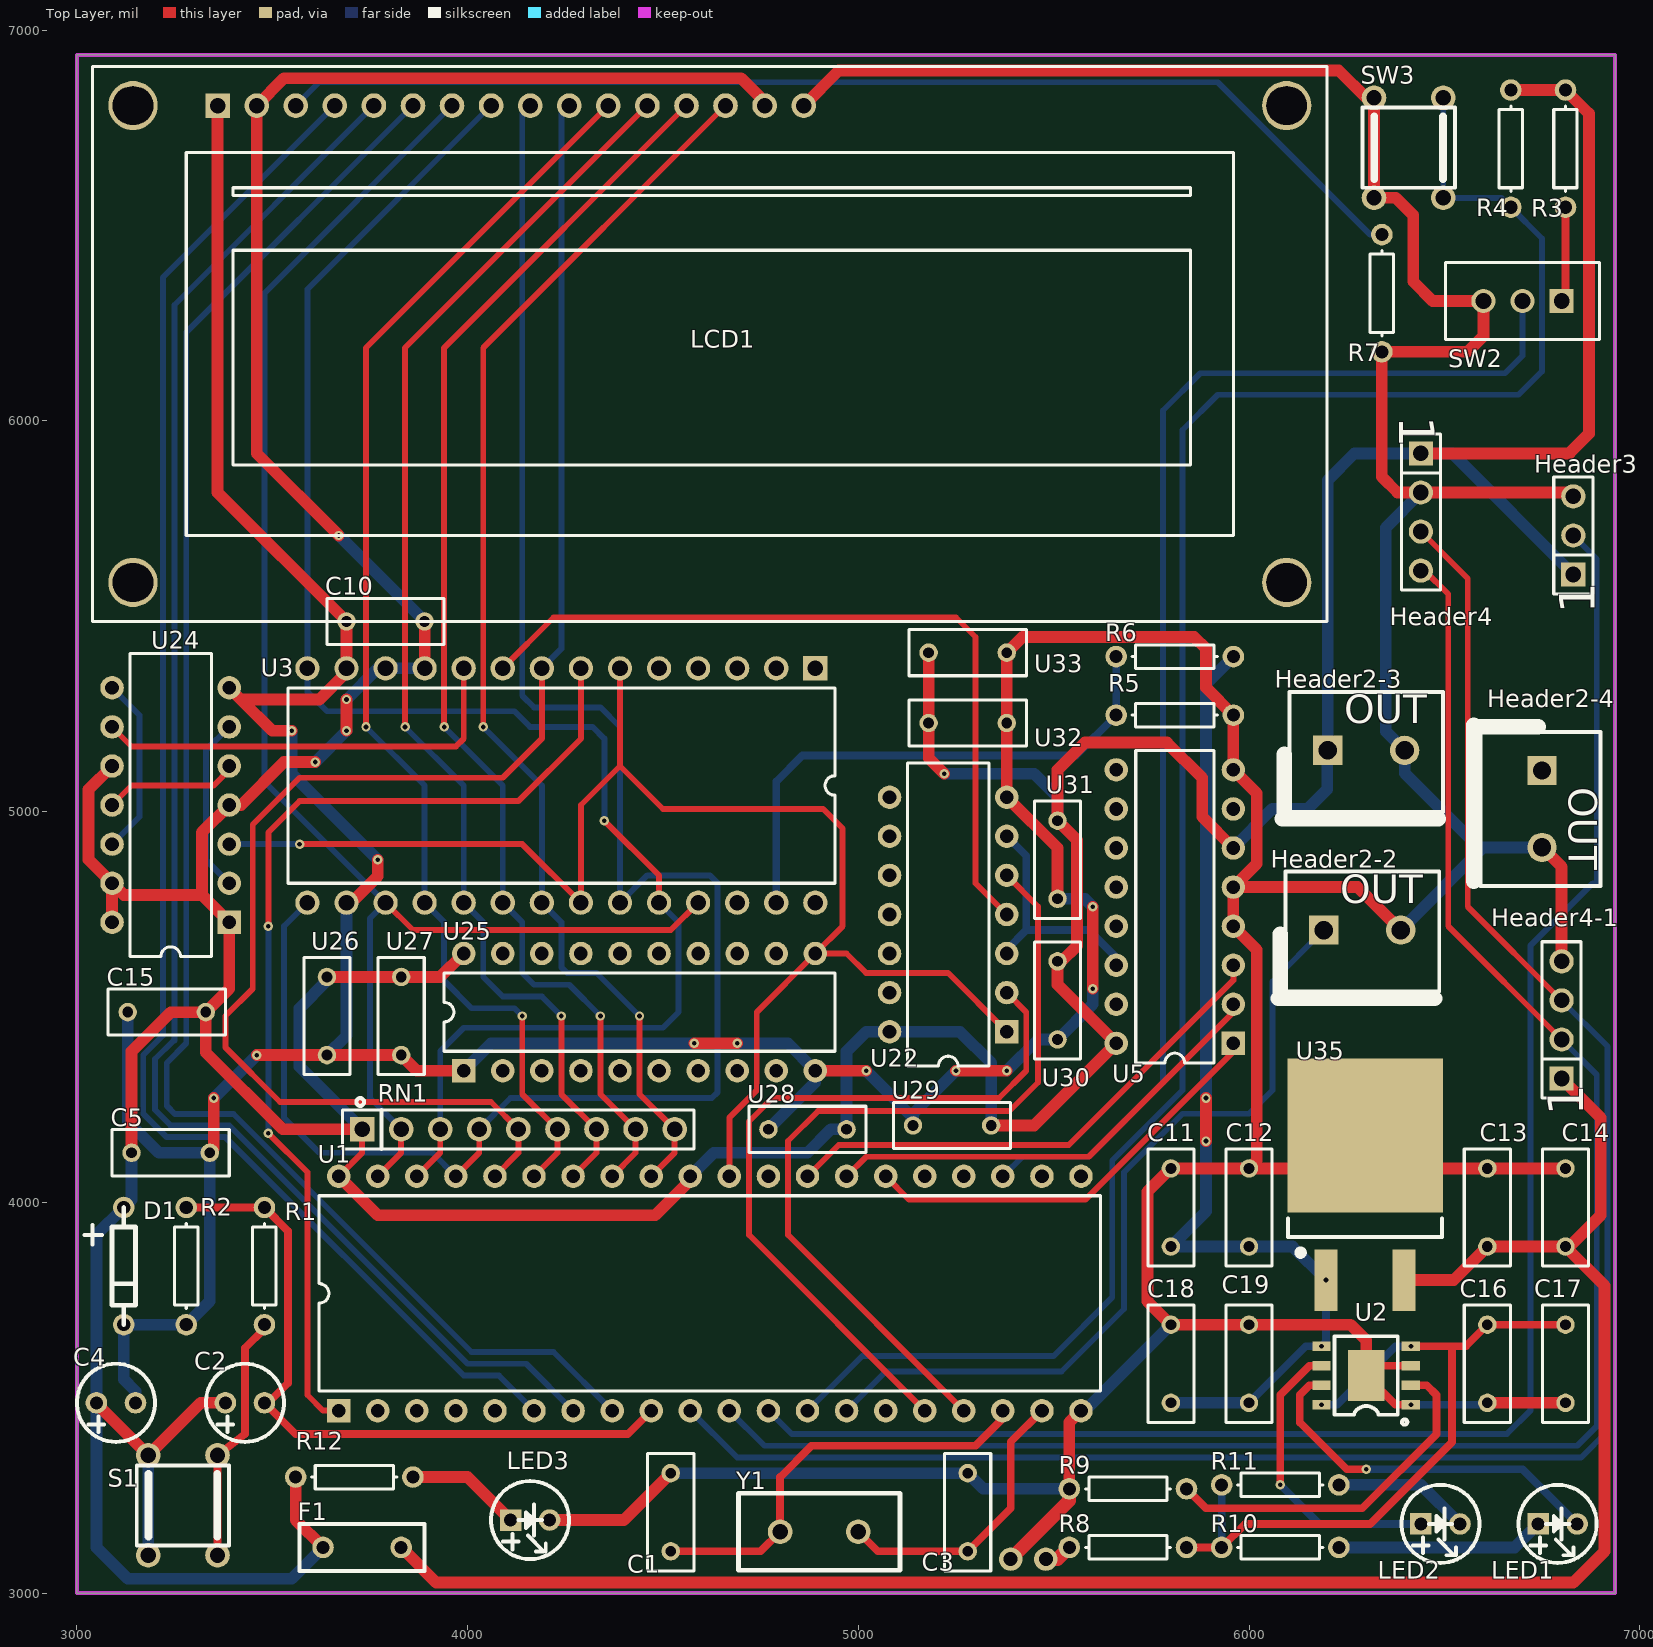
[diagram p0: Top Layer view]
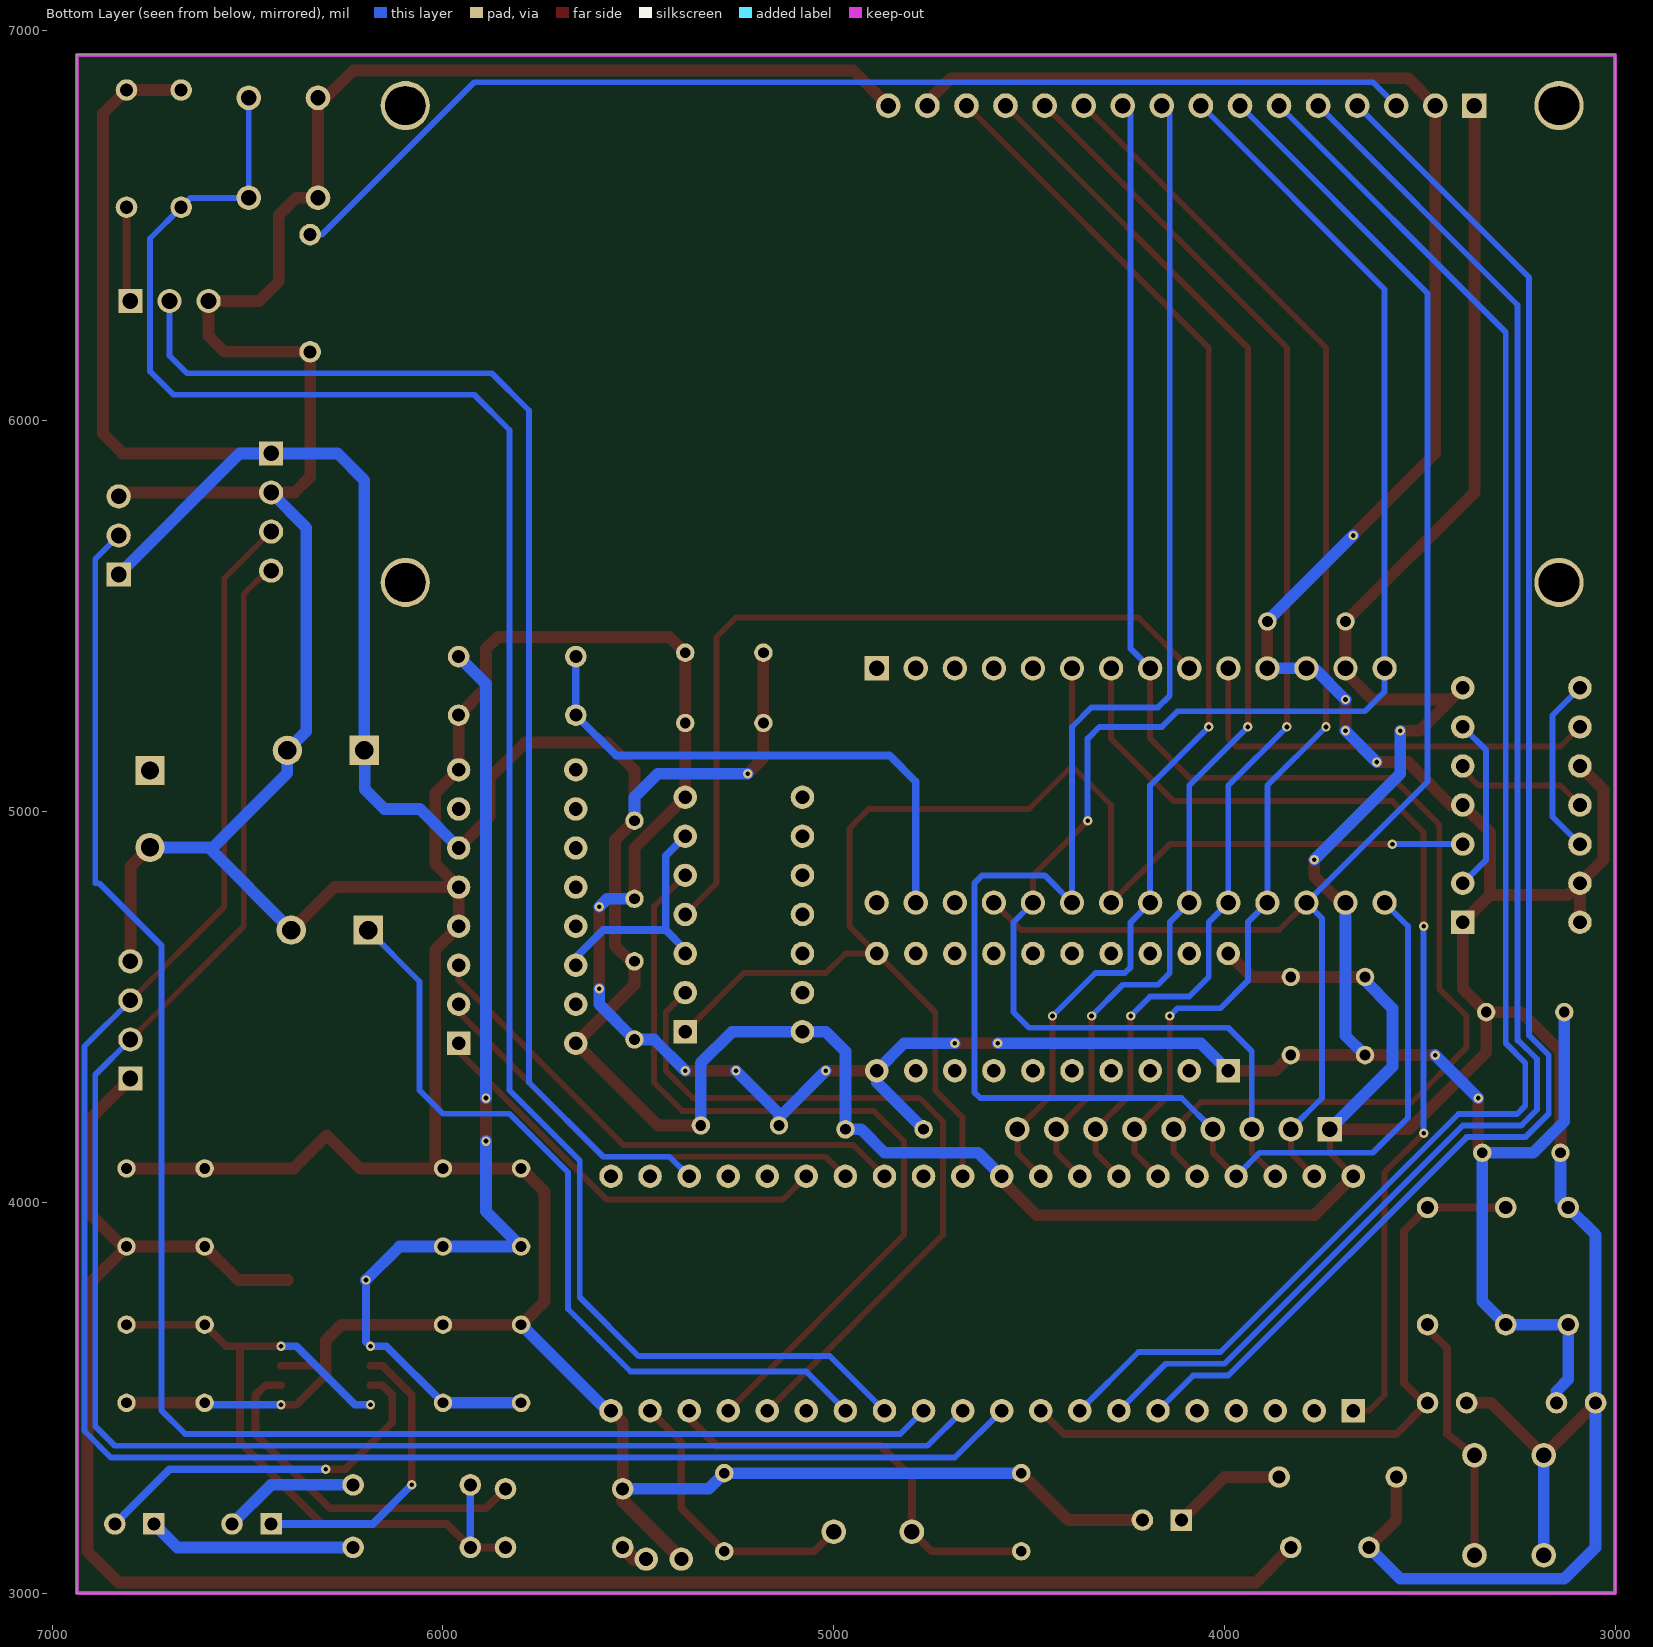
[diagram p1: Bottom Layer view, seen from below]
# Altium PCB MISC52142.pcbdoc
Units mil, origin at the board's own origin, x right, y up, seen from the top; angles counter-clockwise.
Board outline 3937.01 x 3937.01 mil, 2 copper layers (Top Layer, Bottom Layer), stack 62.205 mil thick; 60 components, 49 nets, 285 pads, 37 vias.

## Layer stack, top to bottom
Top Solder Mask Layer: solder mask 0.394, Dk 3.3
Top Layer: signal copper 1.378
Dielectric1: surface 59.449, FR4, Dk 4.5
Bottom Layer: signal copper 1.378
Bottom Solder Mask Layer: solder mask 0.394, Dk 3.3

## Board outline
3000,6937.01 3000,3000 6937.01,3000 6937.01,6937.01

## Design rules (kind name [scope] priority, off if disabled: settings)
BoardOutlineClearance copperThickness2oz_1 [All] p2 off: genericclearance=7.99 ignorepadtopadclearanceinfootprint=FALSE except(0: Arc-SplitContinuation Track-SplitContinuation SMDPad-SplitContinuation THPad-SplitContinuation Via-SplitContinuation Fill-SplitContinuation Region-SplitContinuation Poly-SplitContinuation Text-SplitContinuation Hole-SplitContinuation; 5.98: SMDPad-CutoutEdge THPad-CutoutEdge Via-CutoutEdge Fill-CutoutEdge Region-CutoutEdge Text-CutoutEdge Hole-CutoutEdge; 10: Poly-OutlineEdge Poly-CutoutEdge; 11.81: Arc-OutlineEdge Track-OutlineEdge SMDPad-OutlineEdge THPad-OutlineEdge Via-OutlineEdge Fill-OutlineEdge Region-OutlineEdge Text-OutlineEdge Hole-OutlineEdge Arc-CutoutEdge Track-CutoutEdge)
BoardOutlineClearance Plane_innerPlane_1 [All] p4 off: genericclearance=4.02 ignorepadtopadclearanceinfootprint=FALSE except(0: Arc-SplitContinuation Track-SplitContinuation SMDPad-SplitContinuation THPad-SplitContinuation Via-SplitContinuation Fill-SplitContinuation Region-SplitContinuation Poly-SplitContinuation Text-SplitContinuation Hole-SplitContinuation; 5.98: SMDPad-CutoutEdge THPad-CutoutEdge Via-CutoutEdge Fill-CutoutEdge Region-CutoutEdge Text-CutoutEdge Hole-CutoutEdge; 10: Poly-OutlineEdge Poly-CutoutEdge; 11.81: Arc-OutlineEdge Track-OutlineEdge SMDPad-OutlineEdge THPad-OutlineEdge Via-OutlineEdge Fill-OutlineEdge Region-OutlineEdge Text-OutlineEdge Hole-OutlineEdge Arc-CutoutEdge Track-CutoutEdge)
BoardOutlineClearance Copper_copperRegion_1 [All] p6 off: genericclearance=4.02 ignorepadtopadclearanceinfootprint=FALSE except(0: Arc-SplitContinuation Track-SplitContinuation SMDPad-SplitContinuation THPad-SplitContinuation Via-SplitContinuation Fill-SplitContinuation Region-SplitContinuation Poly-SplitContinuation Text-SplitContinuation Hole-SplitContinuation; 5.98: SMDPad-CutoutEdge THPad-CutoutEdge Via-CutoutEdge Fill-CutoutEdge Region-CutoutEdge Text-CutoutEdge Hole-CutoutEdge; 10: Poly-OutlineEdge Poly-CutoutEdge; 11.81: Arc-OutlineEdge Track-OutlineEdge SMDPad-OutlineEdge THPad-OutlineEdge Via-OutlineEdge Fill-OutlineEdge Region-OutlineEdge Text-OutlineEdge Hole-OutlineEdge Arc-CutoutEdge Track-CutoutEdge)
BoardOutlineClearance copperThickness1oz_1 [All] p8: genericclearance=4.02 ignorepadtopadclearanceinfootprint=FALSE except(0: Arc-SplitContinuation Track-SplitContinuation SMDPad-SplitContinuation THPad-SplitContinuation Via-SplitContinuation Fill-SplitContinuation Region-SplitContinuation Poly-SplitContinuation Text-SplitContinuation Hole-SplitContinuation; 5.98: SMDPad-CutoutEdge THPad-CutoutEdge Via-CutoutEdge Fill-CutoutEdge Region-CutoutEdge Text-CutoutEdge Hole-CutoutEdge; 10: Poly-OutlineEdge Poly-CutoutEdge; 11.81: Arc-OutlineEdge Track-OutlineEdge SMDPad-OutlineEdge THPad-OutlineEdge Via-OutlineEdge Fill-OutlineEdge Region-OutlineEdge Text-OutlineEdge Hole-OutlineEdge Arc-CutoutEdge Track-CutoutEdge)
Clearance copperThickness2oz [All] p1 off: gap=7.99 ignorepadtopadclearanceinfootprint=FALSE except(5.98: SMDPad-Track SMDPad-SMDPad THPad-Track SMDPad-THPad THPad-THPad Track-Via SMDPad-Via THPad-Via Via-Via Fill-Track Region-Track Fill-SMDPad Region-SMDPad Fill-THPad Region-THPad Fill-Via Region-Via Fill-Fill Fill-Region Region-Region Arc-Track Arc-SMDPad Arc-THPad Arc-Via Fill-Arc Region-Arc Arc-Arc Text-Track SMDPad-Text Text-THPad Text-Via Fill-Text Region-Text Arc-Text Text-Text Hole-Track Hole-SMDPad Hole-THPad Hole-Via Fill-Hole Region-Hole Hole-Arc Hole-Text; 10: Poly-Track Poly-SMDPad Poly-THPad Poly-Via Poly-Fill Poly-Region Poly-Poly Poly-Arc Poly-Text Poly-Hole)
Clearance Plane_innerPlane [All] p3 off: gap=4.02 ignorepadtopadclearanceinfootprint=FALSE except(5.98: SMDPad-Track SMDPad-SMDPad THPad-Track SMDPad-THPad THPad-THPad Track-Via SMDPad-Via THPad-Via Via-Via Fill-Track Region-Track Fill-SMDPad Region-SMDPad Fill-THPad Region-THPad Fill-Via Region-Via Fill-Fill Fill-Region Region-Region Arc-Track Arc-SMDPad Arc-THPad Arc-Via Fill-Arc Region-Arc Arc-Arc Text-Track SMDPad-Text Text-THPad Text-Via Fill-Text Region-Text Arc-Text Text-Text Hole-Track Hole-SMDPad Hole-THPad Hole-Via Fill-Hole Region-Hole Hole-Arc Hole-Text; 10: Poly-Track Poly-SMDPad Poly-THPad Poly-Via Poly-Fill Poly-Region Poly-Poly Poly-Arc Poly-Text Poly-Hole)
Clearance Copper_copperRegion [All] p5 off: gap=4.02 ignorepadtopadclearanceinfootprint=FALSE except(5.98: SMDPad-Track SMDPad-SMDPad THPad-Track SMDPad-THPad THPad-THPad Track-Via SMDPad-Via THPad-Via Via-Via Fill-Track Region-Track Fill-SMDPad Region-SMDPad Fill-THPad Region-THPad Fill-Via Region-Via Fill-Fill Fill-Region Region-Region Arc-Track Arc-SMDPad Arc-THPad Arc-Via Fill-Arc Region-Arc Arc-Arc Text-Track SMDPad-Text Text-THPad Text-Via Fill-Text Region-Text Arc-Text Text-Text Hole-Track Hole-SMDPad Hole-THPad Hole-Via Fill-Hole Region-Hole Hole-Arc Hole-Text; 10: Poly-Track Poly-SMDPad Poly-THPad Poly-Via Poly-Fill Poly-Region Poly-Poly Poly-Arc Poly-Text Poly-Hole)
Clearance copperThickness1oz [All] p7: gap=4.02 ignorepadtopadclearanceinfootprint=FALSE except(5.98: SMDPad-Track SMDPad-SMDPad THPad-Track SMDPad-THPad THPad-THPad Track-Via SMDPad-Via THPad-Via Via-Via Fill-Track Region-Track Fill-SMDPad Region-SMDPad Fill-THPad Region-THPad Fill-Via Region-Via Fill-Fill Fill-Region Region-Region Arc-Track Arc-SMDPad Arc-THPad Arc-Via Fill-Arc Region-Arc Arc-Arc Text-Track SMDPad-Text Text-THPad Text-Via Fill-Text Region-Text Arc-Text Text-Text Hole-Track Hole-SMDPad Hole-THPad Hole-Via Fill-Hole Region-Hole Hole-Arc Hole-Text; 10: Poly-Track Poly-SMDPad Poly-THPad Poly-Via Poly-Fill Poly-Region Poly-Poly Poly-Arc Poly-Text Poly-Hole)
DiffPairsRouting differentialPair [All] p1: maxlimit=6 minlimit=6 mostfreqgap=6 toplayer_minwidth=5 toplayer_prefwidth=10 toplayer_maxwidth=100 toplayer_mingap=6 toplayer_prefgap=6 toplayer_maxgap=6 bottomlayer_minwidth=5 bottomlayer_prefwidth=10 bottomlayer_maxwidth=100 bottomlayer_mingap=6 bottomlayer_prefgap=6 bottomlayer_maxgap=6 maxuncoupledlength=10
HoleToHoleClearance otherClearance [All] p1: gap=11.8 allowstackedmicrovias=TRUE
Length netLength [All] p1: minlimit=0 maxlimit=0
PasteMaskExpansion pasteMaskExpansion [All] p1: expansion=0
PlaneConnect innerPlane [All] p1: planeconnectstyle=Relief reliefexpansion=20 reliefentries=4 reliefconductorwidth=10 reliefairgap=10
PolygonConnect copperRegion [All] p1: connectstyle=Relief reliefconductorwidth=10 reliefentries=4 polygonreliefangle="90 Angle" airgapwidth=10 via.connectstyle=Relief via.reliefconductorwidth=10 via.reliefentries=4 via.polygonreliefangle="90 Angle" via.airgapwidth=10
RoutingVias viaSize [All] p1: holewidth=12.01 width=24.02 viastyle="Through Hole" minholewidth=11.81 minwidth=19.68 maxholewidth=248.03 maxwidth=393.7
SolderMaskExpansion solderMaskExpansion [IsVia] p1: expansion=-1000 istentingtop=TRUE
SolderMaskExpansion solderMaskExpansion [All] p2: expansion=2 istentingtop=FALSE
Width copperThickness2oz_2 [All] p1 off: maxlimit=100 minlimit=8 preferedwidth=10
Width copperThickness1oz_2 [All] p2: maxlimit=100 minlimit=5 preferedwidth=10

## Components (designator, comment, footprint, x,y, rotation, side; value= is the part's Value field where it differs from the comment)
C1 "33pF" RAD-0.2 4520,3207.01 r90 top
C2 "10uF" RB1-2 3430,3487.01 r90 top
C3 "33pF" RAD-0.2 5280,3207.01 r90 top
C4 "22uF" RB1-2 3100,3487.01 r90 top
C5 "100nF" RAD-0.2 3240,4127.01 r0 top
C10 "100nF" RAD-0.2 3790,5487.01 r0 top
C11 "100nF" RAD-0.2 5800,3987.01 r270 top
C12 "100nF" RAD-0.2 6000,3987.01 r270 top
C13 "10uF" RAD-0.2 6610,3987.01 r270 top
C14 "10uF" RAD-0.2 6810,3987.01 r270 top
C15 "100nF" RAD-0.2 3230,4487.01 r0 top
C16 "10uF" RAD-0.2 6610,3587.01 r90 top
C17 "100nF" RAD-0.2 6810,3587.01 r90 top
C18 "10uF" RAD-0.2 5800,3587.01 r270 top
C19 "100nF" RAD-0.2 6000,3587.01 r270 top
D1 "1N5819" DIODE-3 3120,3987.01 r180 top
F1 "JK60-050" FUSE-2 3630,3117.01 r0 top
Header2-2 "XY-XHB2.54-2A21" CON2-5 6290,4697.01 r0 top
Header2-3 "XY-XHB2.54-2A21" CON2-5 6300,5157.01 r0 top
Header2-4 "XY-XHB2.54-2A21" CON2-5 6750,5007.01 r270 top
Header3 "PM254V-11-03-H85" CON3 6830,5607.01 r0 top
Header4 "PM254-1-04-W-8.5" CON4 6440,5917.01 r270 top
Header4-1 "PM254-1-04-W-8.5" CON4 6800,4317.01 r90 top
LCD1 "LCM1602K-NSW-BBW" LCD1602 4620,6197.01 r0 top
LED1 "204-10SYGD/S530-E3" LED1 6790,3177.01 r90 top
LED2 "333-2SYGD/S530-E2-L" LED1 6490,3177.01 r90 top
LED3 "204-10SYGD/S530-E3" LED1 4160,3187.01 r90 top
R1 "200Ω" AXIAL-0.3 3480,3687.01 r90 top
R2 "10kΩ" AXIAL-0.3 3280,3987.01 r270 top
R3 "1kΩ" AXIAL-0.3 6810,6547.01 r90 top
R4 "10kΩ" AXIAL-0.3 6670,6547.01 r90 top
R5 "10kΩ" AXIAL-0.3 5960,5247.01 r180 top
R6 "10kΩ" AXIAL-0.3 5660,5397.01 r0 top
R7 "3.5kΩ" AXIAL-0.3 6340,6177.01 r90 top
R8 "250mΩ" AXIAL-0.3 5540,3117.01 r0 top
R9 "1.2kΩ" AXIAL-0.3 5540,3267.01 r0 top
R10 "2kΩ" AXIAL-0.3 5930,3117.01 r0 top
R11 "2kΩ" AXIAL-0.3 5930,3277.01 r0 top
R12 "1kΩ" AXIAL-0.3 3860,3297.01 r180 top
RN1 "4.7kΩ" RP 3730,4187.01 r0 top
S1 "" RST 3360,3097.01 r180 top
SW2 "KH-SS12D01-G3-5.0" RT 6800,6307.01 r90 top
SW3 "" RST 6320,6827.01 r0 top
U1 "STC89C51RC-40I-PDIP40" DIP-40 3670,3467.01 r0 top
U2 "TP4056-42-ESOP8" ESOP-8_L4.9-W3.9-P1.27-LS6.0-BL-EP 6300,3557.01 r90 top
U3 "ADC0809CCV/NOPB" DIP-28 4890,5367.01 r270 top
U5 "74HC138D,653" DIP-16 5960,4407.01 r180 top
U22 "74HC02DRG" DIP-14 5230,4737.01 r90 top
U24 "SN74HC74N" DIP-14 3240,5017.01 r90 top
U25 "74HC573D,653" DIP-20 3990,4337.01 r0 top
U26 "100nF" RAD-0.2 3640,4477.01 r90 top
U27 "100nF" RAD-0.2 3830,4477.01 r90 top
U28 "100nF" RAD-0.2 4870,4187.01 r0 top
U29 "100nF" RAD-0.2 5240,4197.01 r0 top
U30 "100nF" RAD-0.2 5510,4517.01 r90 top
U31 "100nF" RAD-0.2 5510,4877.01 r90 top
U32 "100nF" RAD-0.2 5280,5227.01 r180 top
U33 "100nF" RAD-0.2 5280,5407.01 r180 top
U35 "LM7805S2/TR" TO-263-2_L10.0-W9.1-P5.08-LS15.2-BL 6297.05,3986.36 r0 top
Y1 "11.0592MHz" XTAL-2 4800,3157.01 r0 top

## Footprints (in the part's own frame and the unit in brackets; to place one, negate y for a bottom-side part, rotate by r counter-clockwise, add the part's x,y. Pads: shape width x height; smd on the part's side, far side on the other; paste and mask are expansions set on the pad)
AXIAL-0.3 [mm]
  round 1.4 hole 0.85: 1(0,0) 2(7.62,0)
  silkscreen extent 1.04,-0.76 6.58,0.76
CON2-5 [mil]
  rect 75x75 hole 47: 1(-98.43,0)
  round 75 hole 47: 2(98.43,0)
  silkscreen extent -215,-175 197,150
CON3 [mil]
  rect 62x62 hole 40: 1(0,0)
  round 62 hole 40: 2(0,100) 3(0,200)
  silkscreen extent -50,-50 50,250
CON4 [mil]
  rect 62x62 hole 40: 1(0,0)
  round 62 hole 40: 2(100,0) 3(200,0) 4(300,0)
  silkscreen extent -50,-50 350,50
DIODE-3 [mm]
  round 1.4 hole 0.85: 1(0,0) 2(0,7.62)
  silkscreen extent -0.76,0 2.54,7.62
DIP-14 [mil]
  rect 60x60 hole 35: 1(-300,-150)
  round 60 hole 35: 2(-200,-150) 3(-100,-150) 4(0,-150) 5(100,-150) 6(200,-150) 7(300,-150) 8(300,150) 9(200,150) 10(100,150) 11(0,150) 12(-100,150) 13(-200,150) 14(-300,150)
  silkscreen extent -388,-104 388,104
DIP-16 [mil]
  rect 60x60 hole 35: 1(0,0)
  round 60 hole 35: 2(0,-100) 3(0,-200) 4(0,-300) 5(0,-400) 6(0,-500) 7(0,-600) 8(0,-700) 9(300,-700) 10(300,-600) 11(300,-500) 12(300,-400) 13(300,-300) 14(300,-200) 15(300,-100) 16(300,0)
  silkscreen extent 50,-750 250,50
DIP-20 [mil]
  rect 60x60 hole 35: 1(0,0)
  round 60 hole 35: 2(100,0) 3(200,0) 4(300,0) 5(400,0) 6(500,0) 7(600,0) 8(700,0) 9(800,0) 10(900,0) 11(900,300) 12(800,300) 13(700,300) 14(600,300) 15(500,300) 16(400,300) 17(300,300) 18(200,300) 19(100,300) 20(0,300)
  silkscreen extent -50,50 950,250
DIP-28 [mil]
  rect 62x62 hole 40: 1(0,0)
  round 62 hole 40: 2(0,-100) 3(0,-200) 4(0,-300) 5(0,-400) 6(0,-500) 7(0,-600) 8(0,-700) 9(0,-800) 10(0,-900) 11(0,-1000) 12(0,-1100) 13(0,-1200) 14(0,-1300) 15(600,-1300) 16(600,-1200) 17(600,-1100) 18(600,-1000) 19(600,-900) 20(600,-800) 21(600,-700) 22(600,-600) 23(600,-500) 24(600,-400) 25(600,-300) 26(600,-200) 27(600,-100) 28(600,0)
  silkscreen extent 50,-1350 550,50
DIP-40 [mil]
  rect 60x60 hole 35: 1(0,0)
  round 60 hole 35: 2(100,0) 3(200,0) 4(300,0) 5(400,0) 6(500,0) 7(600,0) 8(700,0) 9(800,0) 10(900,0) 11(1000,0) 12(1100,0) 13(1200,0) 14(1300,0) 15(1400,0) 16(1500,0) 17(1600,0) 18(1700,0) 19(1800,0) 20(1900,0) 21(1900,600) 22(1800,600) 23(1700,600) 24(1600,600) 25(1500,600) 26(1400,600) 27(1300,600) 28(1200,600) 29(1100,600) 30(1000,600) 31(900,600) 32(800,600) 33(700,600) 34(600,600) 35(500,600) 36(400,600) 37(300,600) 38(200,600) 39(100,600) 40(0,600)
  silkscreen extent -50,50 1950,550
ESOP-8_L4.9-W3.9-P1.27-LS6.0-BL-EP [mm]
  rect 0.6x1.2 smd: 1(-1.905,-2.908) 2(-0.635,-2.908) 3(0.635,-2.908) 4(1.905,-2.908) 5(1.905,2.908) 6(0.635,2.908) 7(-0.635,2.908) 8(-1.905,2.908)
  rect 3.3x2.4 smd: 9(0,0)
  silkscreen extent -3.2,-2.67 2.55,2.05
FUSE-2 [mm]
  round 1.4 hole 0.85: 1(0,0) 2(5.08,0)
  silkscreen extent -1.52,-1.52 6.6,1.52
LCD1602 [mm]
  round 3.2 hole 2.5 slot 2.625 at 0 deg: 0(-37.5,-15.5) 0(-37.5,15.5) 0(37.5,-15.5) 0(37.5,15.5)
  rect 1.6x1.6 hole 1: 1(-32,15.5)
  round 1.6 hole 1: 2(-29.46,15.5) 3(-26.92,15.5) 4(-24.38,15.5) 5(-21.84,15.5) 6(-19.3,15.5) 7(-16.76,15.5) 8(-14.22,15.5) 9(-11.68,15.5) 10(-9.14,15.5) 11(-6.6,15.5) 12(-4.06,15.5) 13(-1.52,15.5) 14(1.02,15.5) 15(3.56,15.5) 16(6.1,15.5)
  silkscreen extent -40.13,-18.03 40.13,18.03
LED1 [mm]
  rect 1.4x1.4 hole 0.85: 1(0,1.27)
  round 1.4 hole 0.85: 2(0,-1.27)
  silkscreen extent -2.54,-2.54 2.54,2.54
RAD-0.2 [mm]
  round 1.2 hole 0.7: 1(-2.54,0) 2(2.54,0)
  silkscreen extent -3.81,-1.5 3.81,1.5
RB1-2 [mm]
  round 1.4 hole 0.85: 1(0,1.27) 2(0,-1.27)
  silkscreen extent -2.54,-2.54 2.54,2.54
RP [mm]
  rect 1.6x1.6 hole 1: 1(0,0)
  round 1.6 hole 1: 2(2.54,0) 3(5.08,0) 4(7.62,0) 5(10.16,0) 6(12.7,0) 7(15.24,0) 8(17.78,0) 9(20.32,0)
  silkscreen extent -1.27,-1.27 21.59,2.03
RST [mm]
  round 1.6 hole 1: 1(0,0) 2(0,-6.5) 3(4.5,0) 4(4.5,-6.5)
  silkscreen extent -0.75,-5.84 5.25,-0.63
RT [mil]
  rect 62x62 hole 40: 1(0,0)
  round 62 hole 40: 2(0,100) 3(0,200)
  silkscreen extent -98,-97 98,297
TO-263-2_L10.0-W9.1-P5.08-LS15.2-BL [mm]
  rect 1.5x4 smd: 1(-2.54,-4.7) 3(2.54,-4.7)
  rect 10.1x10 smd: 4(0,4.7)
  silkscreen extent -5,-3.12 5,-0.7
XTAL-2 [mm]
  round 1.6 hole 1: 1(-0.005,0.001) 2(5.075,0.001)
  silkscreen extent -2.71,-2.5 7.79,2.5

## Free pads (board coordinates)
  round 60 hole 36: 41(5390,3087.01) 42(5480,3087.01)

## Via types
v1: diameter 24.02, hole 12, Top Layer to Bottom Layer, 37 vias

## Nets (pads, with @x,y where several pads share a name; then routed paths per layer and width w, separated by ;. In a path a pad name is that pad's centre, name@x,y a point inside that pad or via, vN(x,y) a via of type N, cw(c..) or ccw(c..) an arc to the next point about the centre after c; other vN are vias at no path point)
$1N3565: C1.1 U1.18 Y1.1 | length 1092.7
  Top Layer w20: C1.1 4749.77,3107.01 Y1.1 4799.82,3296.83 4880,3377.01 5300,3377.01 5370,3447.01 U1.18
$1N3571: C3.1 U1.19 Y1.2 | length 739.6
  Top Layer w20: Y1.2 5049.87,3107.01 C3.1 5390,3217.01 5390,3387.01 U1.19
$1N4012: C2.2 R1.2 R2.1 U1.9 | length 1803.6
  Top Layer w20: R2.1 R1.2 3540,3927.01 3540,3537.01 3490,3487.01 C2.2 3560,3407.01 4410,3407.01 U1.9
$1N4197: R1.1 S1.1 S1.2 | length 645.1
  Top Layer w20: S1.1 S1.2 3430,3407.01 3430,3627.01 3480,3677.01 R1.1
$1N12035: U24.2 U24.6 | length 449.7
  Bottom Layer w15: U24.2 3330,4877.01 3330,5157.01 U24.6
$1N12040: U24.5 U24.11 | length 347.3
  Top Layer w15: U24.11 3140,5067.01 3350,5067.01 3390,5107.01 U24.5
$1N12054: U24.8 U24.12 | length 458
  Bottom Layer w15: U24.12 3160,4987.01 3160,5247.01 U24.8
$1N12198: U3.10 U24.9 | length 1109
  Top Layer w15: U24.9 3140,5167.01 3970,5167.01 3990,5187.01 U3.10
$1N12341: R5.2 R6.1 U3.27 | length 1400.4
  Bottom Layer w20: U3.27 4790,5077.01 4856.79,5143.8 5556.79,5143.8 R5.2 R6.1
$1N13639: R3.1 SW2.1 | length 244.1
  Top Layer w20: SW2.1 6810,6317.01 R3.1
$1N18579: R4.1 SW3.3 SW3.4 U1.13 | length 5068.7
  Bottom Layer w15: U1.13 5010,3607.01 5500,3607.01 5650,3757.01 5650,4107.01 5830,4287.01 5830,5977.01 5920,6067.01 6690,6067.01 6750,6127.01 6750,6467.01 R4.1 6645.91,6571.1 SW3.4 SW3.3
$1N23221: Header4-1.2 Header4.4 U1.11 | length 4680.2
  Top Layer w15: Header4.4 6450,5617.01 6510,5557.01 6510,4707.01 Header4-1.2
  Bottom Layer w15: U1.11 4760,3377.01 6840,3377.01 6890,3427.01 6890,4327.01 Header4-1.2 Header4-1.2@6780,4417.01
$1N23232: Header4-1.3 Header4.3 U1.10 | length 4945.6
  Top Layer w15: Header4.3 6560,5597.01 6560,4757.01 Header4-1.3
  Bottom Layer w15: U1.10 4690,3347.01 6850,3347.01 6917.71,3414.72 6917.71,4399.3 Header4-1.3 Header4-1.3@6780,4517.01
$1N24486: LCD1.3 R7.2 | length 2966.1
  Bottom Layer w15: LCD1.3 3619.92,6867.01 5920,6867.01 6310,6477.01 R7.2
$1N29519: U5.14 U22.3 U22.6 | length 620.4
  Bottom Layer w20: U22.3 5380,4647.01 5430,4697.01 ; U22.6 5430,4887.01 5430,4697.01 ; U5.14 5660,4627.01 5590,4697.01 5430,4697.01
$1N30987: R9.2 U2.2 | length 915.3
  Top Layer w20: R9.2 5890,3217.01 6290,3217.01 6480,3407.01 6480,3507.01 6455,3532.01 U2.2
$1N30991: LED1.2 U2.7 | length 953.6
  Top Layer w20: U2.7 6155,3532.01 6130,3507.01 6130,3437.01 6250,3317.01 v1(6300,3317.01)
  Bottom Layer w20: v1(6300,3317.01) 6700,3317.01 LED1.2
$1N30992: LED1.1 R10.2 | length 534.9
  Bottom Layer w30: R10.2 6680,3117.01 LED1.1
$1N30993: LED2.1 U2.6 | length 768
  Top Layer w20: v1(6080,3277.01) 6080,3507.01 6155,3582.01 U2.6
  Bottom Layer w20: v1(6080,3277.01) 6180,3177.01 LED2.1
$1N30994: LED2.2 R11.2 | length 351.4
  Bottom Layer w30: R11.2 6440,3277.01 LED2.2
$1N30996: C16.2 C17.2 R8.2 R10.1 R11.1 U2.4 U2.8 | length 1906
  Top Layer w20: R8.2 R10.1 5990,3177.01 6310,3177.01 6519.5,3386.51 6519.5,3632.01 ; v1(6414.5,3632.01) 6519.5,3632.01 ; C17.2 C16.2 6555,3632.01 6519.5,3632.01
  Bottom Layer w20: R10.1 R11.1 ; v1(6185.5,3482.01) 6225,3482.01 6375,3632.01 v1(6414.5,3632.01)
$1N33639: LED3.1 R12.1 | length 295.6
  Top Layer w30: R12.1 4000,3297.01 LED3.1
$1N33707: SW2.2 U1.23 | length 3347.4
  Bottom Layer w15: U1.23 5420,4117.01 5590,4117.01 5780,4307.01 5780,6027.01 5875,6122.01 6655,6122.01 6700,6167.01 SW2.2
+5V: C13.2 C14.2 F1.2 Header4-1.1 U35.3 | length 4934.8
  Top Layer w30: F1.2 3920,3027.01 6830,3027.01 6910,3107.01 6910,3787.01 C14.2 ; U35.3 6524.31,3801.32 C13.2 C14.2 ; Header4-1.1 6900,4217.01 6900,3967.01 6820,3887.01 C14.2
BAT+: C11.2 C12.2 C18.2 C19.2 R6.2 U2.5 U35.1 | length 2628.5
  Top Layer w30: v1(5890,4157.01) v1(5890,4267.01)
  Bottom Layer w20: C19.2 6145,3632.01 v1(6185.5,3632.01) 6197.05,3643.56 v1(6197.05,3801.32)
  Bottom Layer w30: C18.2 C19.2 ; v1(5890,4157.01) 5890,3977.01 C11.2 C12.2 6111.36,3887.01 v1(6197.05,3801.32) ; v1(5890,4267.01) 5890,5327.01 R6.2
GND: C1.2 C3.2 C4.2 C5.2 C10.1 C11.1 C12.1 C13.1 C14.1 C15.1 C16.1 C17.1 C18.1 C19.1 D1.2 Header2-2.2 Header2-3.2 Header2-4.2 Header3.3 Header4-1.4 Header4.2 LCD1.1 LCD1.16 LED3.2 pad.41 R2.2 R5.1 R7.1 R9.1 SW2.3 SW3.1 SW3.2 U1.20 U2.1 U2.3 U2.9 U3.13 U3.16 U5.4 U5.5 U5.8 U22.7 U24.7 U25.1 U25.10 U26.1 U27.1 U28.1 U29.1 U30.1 U31.1 U32.1 U33.1 U35.4 | length 21092.5
  Top Layer w20: v1(6414.5,3482.01) 6375,3482.01 U2.9 6325,3582.01 U2.3
  Top Layer w30: C5.2 3350,4137.01 v1(3350,4267.01) ; LCD1.1 3360.16,5816.85 C10.1 U3.13 3690,5357.01 3620,5287.01 3420,5287.01 ; U24.7 3420,5287.01 ; v1(3460,4377.01) U26.1 U27.1 3870,4337.01 U25.1 ; v1(3550,5207.01) 3500,5207.01 3420,5287.01 ; U3.16 3702.43,4767.01 3770,4834.58 v1(3770,4877.01) ; LED3.2 4400,3187.01 C1.2 ; v1(4580,4407.01) v1(4690,4407.01) ; LCD1.16 4949.92,6897.01 6230,6897.01 6300,6827.01 SW3.1 SW3.2 6375.91,6571.1 6420,6527.01 6420,6357.01 6470,6307.01 SW2.3 6600,6217.01 6560,6177.01 R7.1 6340,5857.01 6380,5817.01 Header4.2 6820,5817.01 Header3.3 ; U25.10 v1(5020,4337.01) ; v1(5250,4337.01) v1(5380,4337.01) ; U31.1 5510,4907.01 U22.7 U32.1 U33.1 5420,5447.01 5860,5447.01 5890,5417.01 5890,5317.01 R5.1 U5.8 6020,5047.01 6020,4867.01 U5.5 ; R9.1 5540,3437.01 U1.20 ; v1(5600,4547.01) v1(5600,4757.01) ; U2.9 6300,3647.01 6260,3687.01 C19.1 C18.1 5740,3747.01 5740,4027.01 C11.1 C12.1 ; Header2-2.2 6278.43,4807.01 U5.5 ; C16.1 C17.1 ; Header2-4.2 6800,4858.58 Header4-1.4 ; C14.1 C13.1 6381.45,4087.01 U35.4 6212.68,4087.01 C12.1 ; U5.5 U5.4 6020,4647.01 6020,4107.01 C12.1
  Top Layer w35: pad.41 5540,3237.01 R9.1
  Bottom Layer w20: v1(6414.5,3482.01) 6605,3482.01 C16.1
  Bottom Layer w30: C15.1 3130,4207.01 3210,4127.01 C5.2 3340,3747.01 R2.2 D1.2 3120,3547.01 3150,3517.01 C4.2 ; v1(3350,4267.01) v1(3460,4377.01) ; v1(3550,5207.01) 3550,5097.01 v1(3770,4877.01) ; U26.1 3690,4427.01 U3.16 ; U25.1 4060,4407.01 v1(4580,4407.01) ; C1.2 C3.2 5320,3267.01 R9.1 ; v1(4690,4407.01) 4820,4407.01 U25.10 4890,4307.01 U28.1 ; v1(5020,4337.01) U29.1@5140,4217.01 ; U29.1 U29.1@5140,4217.01 ; v1(5250,4337.01) 5140,4227.01 U29.1@5140,4217.01 ; v1(5380,4337.01) 5460,4417.01 U30.1 5600,4507.01 v1(5600,4547.01) ; U31.1 5580,4777.01 v1(5600,4757.01) ; U1.20 5580,3467.01 C18.1 ; Header2-2.2 6600,4908.58 ; Header4.2 6350,5727.01 6350,5205.43 Header2-3.2 6398.43,5098.58 6588.43,4908.58 6600,4908.58 ; Header2-4.2 6600,4908.58
IN+: pad.42 R8.1 | length 72.4
  Top Layer w35: pad.42 5510,3087.01 R8.1
P0.0: LCD1.7 RN1.2 U1.39 U3.17 U3.25 | length 4000.1
  Top Layer w15: U1.39 3830,4127.01 RN1.2 ; U3.17 3860,4697.01 4520,4697.01 U3.25
  Bottom Layer w15: RN1.2 3750,4267.01 3750,4727.01 U3.17 3480,5077.01 3480,6327.09 LCD1.7
P0.1: LCD1.8 RN1.3 U1.38 U3.14 U3.24 | length 4279.7
  Top Layer w15: U1.38 3930,4127.01 RN1.3 ; v1(4350,4977.01) 4490,4837.01 U3.24
  Bottom Layer w15: RN1.3 3930,4387.01 3990,4447.01 4500,4447.01 4540,4487.01 4540,4717.01 U3.24 ; LCD1.8 3590,6337.09 U3.14 3590,5307.01 3640,5257.01 4120,5257.01 4160,5217.01 4320,5217.01 4350,5187.01 v1(4350,4977.01)
P0.2: LCD1.9 RN1.4 U1.37 U3.15 U3.23 | length 4945.2
  Top Layer w15: U1.37 4030,4127.01 RN1.4
  Bottom Layer w15: U3.15 3530,4707.01 3530,4217.01 3620,4127.01 3910,4127.01 U1.37 ; RN1.4 4110,4267.01 4625,4267.01 4640,4282.01 4640,4817.01 4620,4837.01 4460,4837.01 U3.23 4390,5217.01 4340,5267.01 4170,5267.01 4140,5297.01 4140,6787.09 LCD1.9
P0.3: LCD1.10 RN1.5 U1.36 U3.8 | length 4061.3
  Top Layer w15: U1.36 4130,4127.01 RN1.5 4060,4257.01 3520,4257.01 3380,4397.01 3380,4477.01 3450,4547.01 3450,4967.01 3570,5087.01 4090,5087.01 4190,5187.01 U3.8
  Bottom Layer w15: U3.8 4240,5417.01 4240,6787.09 LCD1.10
P0.4: LCD1.11 RN1.6 U1.35 U3.18 | length 3289.4
  Top Layer w15: v1(3740,5217.01) 3740,6187.09 LCD1.11 ; v1(4140,4477.01) 4140,4277.01 RN1.6 4230,4127.01 U1.35
  Bottom Layer w15: v1(3740,5217.01) 3890,5067.01 U3.18 3940,4717.01 3940,4567.01 4010,4497.01 4120,4497.01 v1(4140,4477.01)
P0.5: LCD1.12 RN1.7 U1.34 U3.19 | length 3283.5
  Top Layer w15: v1(3840,5217.01) 3840,6187.09 LCD1.12 ; v1(4240,4477.01) 4240,4277.01 RN1.7 4330,4127.01 U1.34
  Bottom Layer w15: v1(3840,5217.01) 3990,5067.01 U3.19 4040,4717.01 4040,4577.01 4090,4527.01 4190,4527.01 v1(4240,4477.01)
P0.6: LCD1.13 RN1.8 U1.33 U3.20 | length 3277.7
  Top Layer w15: v1(3940,5217.01) 3940,6187.09 LCD1.13 ; v1(4340,4477.01) 4340,4277.01 RN1.8 4430,4127.01 U1.33
  Bottom Layer w15: v1(3940,5217.01) 4090,5067.01 U3.20 4140,4717.01 4140,4587.01 4170,4557.01 4260,4557.01 v1(4340,4477.01)
P0.7: LCD1.14 RN1.9 U1.32 U3.21 | length 3268.9
  Top Layer w15: v1(4040,5217.01) 4040,6187.09 LCD1.14 ; v1(4440,4477.01) 4440,4277.01 RN1.9 4530,4127.01 U1.32
  Bottom Layer w15: v1(4040,5217.01) 4190,5067.01 U3.21 4240,4717.01 4240,4602.01 4255,4587.01 4330,4587.01 v1(4440,4477.01)
P1.0: U1.1 U3.7 | length 2657.4
  Top Layer w15: v1(3490,4177.01) 3590,4077.01 3590,3507.01 3630,3467.01 U1.1 ; v1(3490,4707.01) 3490,4947.01 3570,5027.01 4130,5027.01 4290,5187.01 U3.7
  Bottom Layer w15: v1(3490,4177.01) v1(3490,4707.01)
P1.5: LCD1.4 U1.6 | length 4098.1
  Bottom Layer w15: LCD1.4 3220.11,6367.2 3220.11,4427.12 3170,4377.01 3170,4227.01 3230,4167.01 3380,4167.01 3990,3557.01 4080,3557.01 U1.6
P1.6: LCD1.5 U1.7 | length 4192.6
  Bottom Layer w15: LCD1.5 3250,6297.09 3250,4414.56 3247.55,4414.56 3200,4367.01 3200,4237.01 3240,4197.01 3390,4197.01 4000,3587.01 4150,3587.01 U1.7
P1.7: LCD1.6 U1.8 | length 4284.3
  Bottom Layer w15: 3280,6227.01 3280,4407.01 3230,4357.01 3230,4247.01 3250.81,4226.2 3400.81,4226.2 4010,3617.01 4220,3617.01 U1.8 ; 3280,6227.09 LCD1.6
P2.5: U1.26 U5.1 | length 1093
  Top Layer w15: U1.26 5130,4007.01 5581.21,4007.01 5960,4385.79 U5.1
P2.6: U1.27 U5.2 | length 1184
  Top Layer w15: U1.27 5020,4117.01 5590,4117.01 5960,4487.01 U5.2
P2.7: U1.28 U5.3 | length 1336.2
  Top Layer w15: U1.28 4950,4147.01 5538.48,4147.01 5960,4568.53 U5.3
PWM: Header2-2.1 U1.14 | length 2099.2
  Bottom Layer w15: U1.14 5070,3567.01 5520,3567.01 5680,3727.01 5680,4077.01 5830,4227.01 6000,4227.01 6060,4287.01 6060,4565.43 Header2-2.1
R2: U3.9 U22.4 | length 2027.7
  Top Layer w15: U3.9 4220,5497.01 5250,5497.01 5300,5447.01 5300,4817.01 U22.4
RD: U1.17 U22.5 | length 2141.7
  Top Layer w15: U1.17 4820,3917.01 4820,4157.01 4897.12,4234.13 5387.12,4234.13 5460,4307.01 5460,4757.01 U22.5
REDOUT: Header3.2 U1.12 | length 4340.8
  Bottom Layer w15: U1.12 4830,3407.01 6660,3407.01 6720,3467.01 6720,4657.01 6880,4817.01 6890,4817.01 6890,5647.01 Header3.2
VCC: C2.1 C4.1 C5.1 C10.2 C15.2 D1.1 F1.1 Header2-3.1 Header3.1 Header4.1 LCD1.2 LCD1.15 R3.2 R4.2 R12.2 RN1.1 S1.3 S1.4 U1.31 U1.40 U3.11 U3.12 U5.6 U5.16 U22.14 U24.1 U24.4 U24.10 U24.13 U24.14 U25.20 U26.2 U27.2 U28.2 U29.2 U30.2 U31.2 U32.2 U33.2 | length 17824.6
  Top Layer w15: U1.40 3730,4127.01 RN1.1
  Top Layer w30: C4.1 3050,3485.75 S1.4 3316.93,3487.01 C2.1 ; U24.14 U24.13 ; U24.10 3030,5057.01 3030,4877.01 U24.13 ; C5.1 3140,4387.01 3240,4487.01 C15.2 ; R12.2 3560,3187.01 F1.1 ; v1(3610,5127.01) 3530,5127.01 3420,5017.01 U24.4 3320,4947.01 3320,4787.01 ; U26.2 U27.2 3930,4577.01 U25.20 ; U1.40 3770,3967.01 4480,3967.01 4570,4057.01 U1.31 ; v1(3670,5707.01) 3460.16,5916.85 LCD1.2 3529.92,6877.01 4700,6877.01 4760.16,6816.85 LCD1.15 ; v1(3690,5207.01) v1(3690,5287.01) ; RN1.1 3526.68,4187.01 3330,4383.69 C15.2 ; U3.11 C10.2 ; U33.2 U32.2 5180,5137.01 v1(5220,5097.01) ; U29.2 5450,4197.01 U5.16 5510,4557.01 U30.2 5520,4617.01 5560,4657.01 5560,4927.01 U31.2 5510,5107.01 5580,5177.01 5790,5177.01 5880,5087.01 5880,4987.01 U5.6 ; Header4.1 6820,5917.01 6870,5967.01 6870,6787.01 R3.2 R4.2 ; U24.13 3120,4787.01 3320,4787.01 ; 3320,4787.01 U24.1 3390,4547.01 C15.2
  Bottom Layer w30: C5.1 3140,4007.01 D1.1 3050,3917.01 C4.1 3050,3117.01 3130,3037.01 3550,3037.01 F1.1 ; S1.3 S1.4 ; v1(3610,5127.01) v1(3690,5207.01) ; U26.2 3640,4567.01 3570,4497.01 3570,4347.01 RN1.1 ; v1(3670,5707.01) C10.2 ; v1(3690,5287.01) 3770,5367.01 U3.12 U3.11 ; U1.31 4630,4127.01 4870,4127.01 4930,4187.01 U28.2 4970,4387.01 5020,4437.01 U22.14 5260,4437.01 5340,4357.01 U29.2 ; v1(5220,5097.01) 5450,5097.01 5510,5037.01 U31.2 ; U5.6 6060,5007.01 6150,5007.01 6200,5057.01 6200,5155.43 Header2-3.1 6201.57,5848.58 6270,5917.01 Header4.1 6520,5917.01 Header3.1
W2: U1.30 U3.6 U3.22 U22.1 U24.3 U25.11 | length 3822.8
  Top Layer w15: v1(3570,4917.01) 4140,4917.01 U3.22 4290,5017.01 4390,5117.01 ; U3.6 4390,5117.01 ; U1.30 4670,4217.01 4740,4287.01 4740,4487.01 U25.11 ; U22.1 5230,4587.01 5020,4587.01 4970,4637.01 U25.11 ; 4390,5117.01 4500,5007.01 4910,5007.01 4960,4957.01 4960,4707.01 U25.11
  Bottom Layer w15: U24.3 v1(3570,4917.01)
WR: U1.16 U22.2 | length 1911
  Top Layer w15: U1.16 4720,3917.01 4720,4207.01 4780,4267.01 5360,4267.01 5430,4337.01 5430,4487.01 U22.2
pads on no net: Header2-4.1 LCD1.0 U1.2 U1.3 U1.4 U1.5 U1.15 U1.21 U1.22 U1.24 U1.25 U1.29 U3.1 U3.2 U3.3 U3.4 U3.5 U3.26 U3.28 U5.7 U5.9 U5.10 U5.11 U5.12 U5.13 U5.15 U22.8 U22.9 U22.10 U22.11 U22.12 U22.13 U25.2 U25.3 U25.4 U25.5 U25.6 U25.7 U25.8 U25.9 U25.12 U25.13 U25.14 U25.15 U25.16 U25.17 U25.18 U25.19

## Keep-outs
Board Outline Layer:
  the board outline again, w10